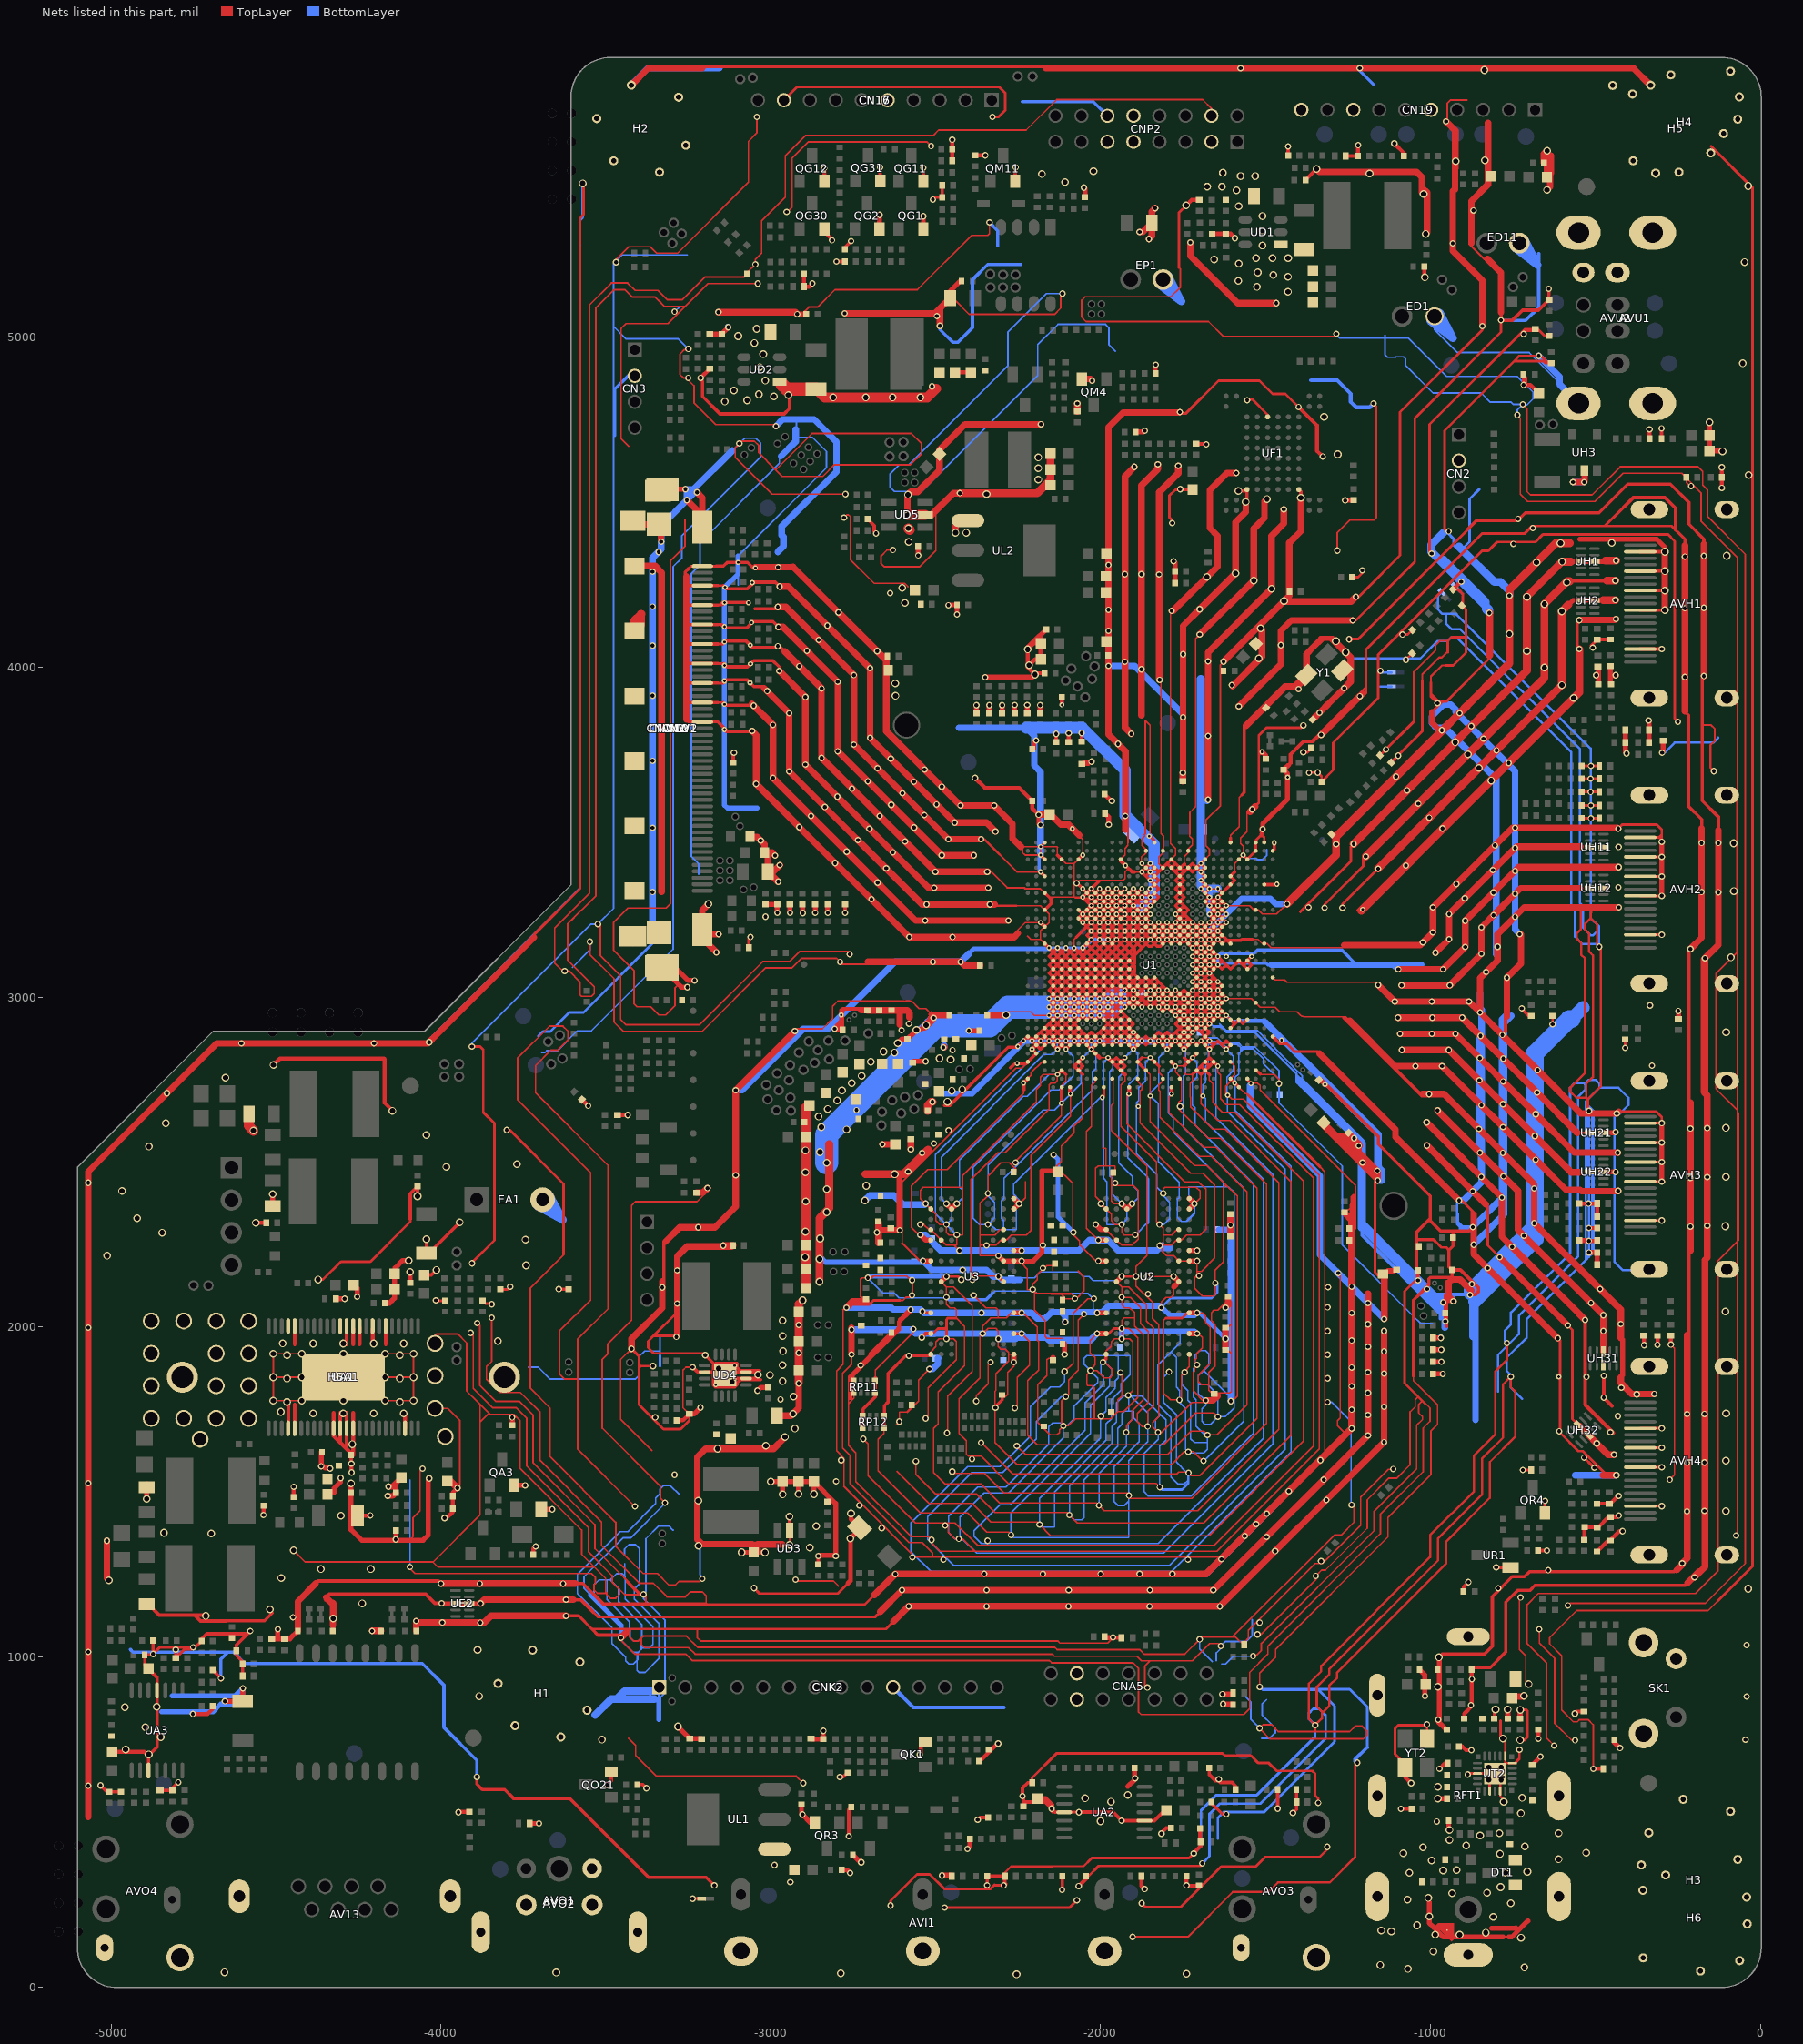
[diagram p0: the nets of this part, all layers, seen from the top]
# Altium PCB MISC86290.PcbDoc (part 17 of 31)
Units mil, origin at the board's own origin, x right, y up, seen from the top; angles counter-clockwise.
Board outline 5104.71 x 5851.49 mil, 2 copper layers (TopLayer, BottomLayer), stack 61.855 mil thick; 1026 components, 667 nets, 4280 pads, 2294 vias.

## Via types
v1: diameter 19.68, hole 11.81, TopLayer to BottomLayer, tented both sides, 1189 vias
v2: diameter 19.68/19.68 (per signal layer), hole 11.81, TopLayer to BottomLayer, tented both sides, 366 vias
v3: diameter 15.75, hole 7.87, TopLayer to BottomLayer, tented both sides, 348 vias
v4: diameter 23.62, hole 15.75, TopLayer to BottomLayer, tented both sides, 309 vias
v5: diameter 15.75/15.75 (per signal layer), hole 7.87, TopLayer to BottomLayer, tented both sides, 59 vias
v6: diameter 24/24 (per signal layer), hole 16, TopLayer to BottomLayer, tented both sides, 23 vias

## Nets (pads, with @x,y where several pads share a name; then routed paths per layer and width w, separated by ;. In a path a pad name is that pad's centre, name@x,y a point inside that pad or via, vN(x,y) a via of type N, cw(c..) or ccw(c..) an arc to the next point about the centre after c; other vN are vias at no path point) (continued)
GND: (continued)
  TopLayer w10: v1(-5032,610) -5012.67,590.67 DO32.A@-5006.75,590.67 ; DO32.A@-5008.83,590.67 DO32.A@-5006.75,590.67 ; RO40.1@-4969.75,590.67 DO32.A@-5006.75,590.67 ; CA14.2@-4892,1159.97 -4887.97,1159.97 -4854.5,1126.5 -4747,1126.5 ; UA3.10@-4886.51,638.49 UA3.10@-4886.51,655.21 -4886.51,699.26 -4887.25,700 -4860.92,726.33 UA3.4@-4860.92,898.32 -4860.92,937.73 CO41.2@-4887.19,964 -4897.27,974.08 -4897.27,1006 v1@-4875,1006 ; RO43.1@-4872.52,1053 RO43.1@-4872.52,1049 v1(-4872.52,1008.48) -4852,1029 v1(-4751.25,1029) ; DO31.A@-4851.5,594.73 RO39.1@-4813.5,594.73 -4813.5,602.63 -4796.63,619.5 v1(-4796.5,619.5) ; v1(-4804,1022) -4803.84,1021.84 CA53.1@-4803.84,996.73 -4776.57,1024 -4756.25,1024 v1(-4751.25,1029) ; v4(-4713,1124) -4715.5,1126.5 -4747,1126.5 ; CO32.1@-4691.78,959.49 -4668,935.71 -4668,930 -4667,931 v1(-4667,935) ; DE1.A@-4601,941.4 CE8.1@-4601,978.37 -4601,985.06 -4620.23,1004.29 CE7.1@-4620.23,1018.5 -4620.23,1035.77 -4586,1070 ; v1(-4578,1078) -4586,1070 ; -4511.68,1132.68 -4534.78,1109.59 -4647.98,1109.59 -4649.08,1108.5 -4729,1108.5 -4747,1126.5 ; -4379.78,1222.16 -4371.94,1230 -4007.84,1230 v2(-4000,1222.16) ; -4093,2326.45 -4093,2404.27 CA35.2@-4071,2426.27 v4(-4071,2396.54) ; CA10.1@-4051,2157.81 -4029.19,2157.81 v4(-4014,2173) ; v4(-4043.95,2265.95) CA30.1@-4043.95,2223.94 -4036.06,2223.94 v4(-3943,2317) ; v1(-3891,636) -3891,614 -3875,598 -3807,598 -3780,571 -3609.66,571 -3370.66,332 -3196.16,332 v2(-3171.25,307.09) ; v1(-3642.77,2114.77) CO24.1@-3613,2114.77 ; v2(-3621.16,1124.16) -3582.16,1124.16 -3564.25,1106.25 ; -3598,1173.16 -3576,1173.16 -3537.67,1134.83 ; -3593.16,1222.16 -3569.85,1222.16 -3507.19,1159.5 -3380.94,1159.5 -3196,1159.5 ; -3542.5,1084.5 -3524,1066 -3462.25,1066 v1(-3454.25,1058) ; v1(-3495.94,611.55) -3483.5,623.99 QO21.E@-3483.5,649.5 ; CO25.1@-3405.05,614.28 CO25.1@-3405.05,612.5 -3387.5,612.5 v1(-3377,602) v1@-3376.5,602.5 ; -3329,2138.75 -3324,2143.75 -3324,2253.75 -3319.25,2258.5 ; -3259.25,4279 -3259.25,4289.33 -3249,4299.57 ; v1(-3237.25,1878) -3222.78,1863.53 UD4.6@-3217.56,1863.53 ; v1@-3215.25,4875 -3207.5,4867.25 -3207.5,4821.44 -3154.06,4768 -2959.5,4768 -2943.5,4784 v4@-2943.5,4824.11 ; -3208,5815.96 -3203,5820.96 v1@-1575,5820.96 ; UD4.6@-3201,1863.53 -3173.28,1863.53 ; -3165,4306.65 -3143.59,4306.65 -3132.25,4318 -3113,4318 ; -3159.77,3834.21 -3130.56,3805 ; -3154.7,4188.54 -3146.25,4197 -3083.5,4197 ; -3149.74,4129.49 -3139.97,4119.72 -3072.53,4119.72 ; UD4.EPAD@-3147.85,1863.53 -3173.28,1863.53 ; -3146.81,4070.43 -3137.25,4080 -3075.25,4080 -3054.75,4059.5 ; v3@-3143.85,4247.6 -3134.08,4237.83 -3071.1,4237.83 -3050.93,4258 -3042.5,4258 ; v3@-3143.52,3893.27 -3135.25,3885 v1@-3061.25,3885 ; v3@-3143.22,3952.32 -3132.94,3962.61 -3072.64,3962.61 ; v3@-3142.63,4011.38 -3132.86,4001.61 -3070.64,4001.61 ; v3@-3141,3815.44 -3130.56,3805 ; v3(-3140.74,3811.12) -3134.62,3805 -3110,3805 ; UD4.EPAD@-3128.17,1843.85 UD4.14@-3075.02,1843.85 -3050.15,1843.85 v4(-3039,1855) -3047.53,1863.53 UD4.15@-3075.02,1863.53 UD4.15@-3089.47,1863.53 ; UD4.EPAD@-3128.17,1863.53 UD4.15@-3089.47,1863.53 ; RW415.1@-3114,3711.73 -3114,3739 v1(-3112,3741) ; v3(-3099.25,4318) -3113,4318 ; v3@-3068.25,4197 -3083.5,4197 ; v3(-3068,4195.5) -3069.5,4197 -3083.5,4197 ; RW73.2@-3066.27,3150 -3066.27,3177.23 v1(-3061.5,3182) ; v3(-3063.01,3952.99) -3072.64,3962.61 ; v3(-3062.2,4066.95) -3054.75,4059.5 ; v3(-3061.62,4010.62) -3070.64,4001.61 ; v3(-3058.19,4135.63) -3058.19,4134.06 -3072.53,4119.72 ; v1(-3057,3807) -3059,3805 -3110,3805 ; v3(-3056.37,4256.63) -3054.99,4258 -3042.5,4258 ; -3048.75,4177.5 v1@-2981.25,4177.5 ; v3(-3047,4301.5) -3045.5,4300 -3029,4300 ; -3033.2,1867.7 -3093.65,1867.7 ; -3031.17,1839.67 -3093.65,1839.67 -3102.73,1830.59 -3102.73,1825.5 -3109.82,1818.41 -3168,1818.41 -3173.28,1823.7 -3173.28,1863.53 ; -3020.25,3937 -3024.75,3941.5 -3051.53,3941.5 -3072.64,3962.61 ; v1(-2977.25,4122) -2993.75,4138.5 -3053.75,4138.5 -3072.53,4119.72 ; v1(-2974.31,3989.07) -2974.31,4000.94 -2993.87,4020.5 -3051.75,4020.5 -3070.64,4001.61 ; v1(-2973.25,4245) -2986.25,4258 -3042.5,4258 ; -2957.85,4047.4 -2969.95,4059.5 -3054.75,4059.5 ; -2932.52,4304 -2933.02,4303.5 -2936.52,4300 -3029,4300 ; v1(-2790.69,635.88) -2780.73,635.88 -2767.34,649.27 CK1.1@-2766,649.27 ; RG40.1@-2775.73,5267 -2775.73,5272.77 v1(-2756.5,5292) ; v1(-2764,456) -2764,536.98 CR5.1@-2755.98,545 ; RD55.1@-2706.7,4449.79 -2686.75,4429.83 -2686.75,4411.5 v1(-2681.25,4406) ; -2639.15,1963.32 -2612.22,1990.25 -2612.22,1998.03 ; -2622.22,1988.03 -2612.22,1998.03 ; -2607.06,2021.8 -2612.22,2016.63 -2612.22,1998.03 ; v2(-2542.64,1968.11) -2530.83,1979.92 U3.P1@-2515.08,1979.92 ; v1@-2502.16,5424.84 RG4.1@-2480.98,5424.84 CG1.1@-2480.98,5463.84 ; -2472.97,2672.03 -2457.97,2672.03 ; -2456.72,2672.03 -2280.72,2848.03 -2253.27,2848.03 v3(-2251.3,2850) v3(-2233.58,2867.72) U1.G30@-2220.79,2880.51 v3(-2207.99,2867.72) ; v1(-2373,506) -2366,513 RO30.1@-2341.73,513 ; v1(-2344.27,307.54) CI1.1@-2344.27,334.99 DI2.A@-2290.73,335 v1@-2290.73,310.35 ; v2@-2320.2,1757.54 -2298.21,1779.53 -2298.94,1780.25 C50.2@-2298.94,1787.48 ; -2273.18,2785.76 -2260.12,2798.82 -2225.71,2798.82 -2208.26,2816.26 ; v3(-2253.27,2798.82) v3@-2251.3,2796.85 ; CO18.2@-2234,546.73 -2234,559.73 ; U1.D30@-2220.79,2803.74 -2208.26,2816.26 ; RO57.1@-2207.96,618.5 -2220.82,618.5 -2237,602.32 v1(-2237,578) -2234,575 -2234,559.73 ; U1.G29@-2195.2,2880.51 U1.F28@-2169.61,2854.92 v3(-2156.81,2867.72) ; v3(-2182.4,3379.53) U1.AF28@-2169.61,3366.73 ; v3(-2182.4,3430.71) U1.AH28@-2169.61,3417.91 ; U1.H28@-2169.61,2906.1 v3(-2131.22,2867.72) ; U1.V28@-2169.61,3162.01 -2131.22,3123.62 ; U1.AB28@-2169.61,3264.37 -2150.91,3283.07 -2150.91,3294.88 -2150.91,3296.85 -2156.81,3302.76 U1.AD28@-2169.61,3315.55 ; v3@-2154.8,3147.65 -2145.22,3138.06 -2145.22,3135.22 ; -2138,529 -2148.66,539.66 -2168.73,559.73 -2234,559.73 ; v5(-2131.22,2765.35) U1.C26@-2118.43,2778.15 -2105.63,2765.35 ; -2130.79,3430.28 U1.AH26@-2118.43,3417.91 ; v3@-2129.21,3147.65 -2129.21,3147.2 -2118.43,3136.42 ; v1@-2116.54,294.46 RI4.1@-2116.54,335 ; v3@-2104,3148 -2093.13,3137.13 -2093.13,3136.13 ; -2073.84,3182.16 -2028.08,3227.92 v3@-2026.92,3227.92 ; v1(-2073.03,3344.98) -2071.09,3344.98 v3(-2054.45,3328.35) U1.AD23@-2041.65,3315.55 -1875.32,3149.21 ; U1.C24@-2067.24,2778.15 -2054.45,2790.94 U1.D24@-2067.24,2803.74 ; U1.H24@-2067.24,2906.1 v3(-2105.63,2867.72) ; U1.J24@-2067.24,2931.69 -2156.81,3021.26 U1.AE15@-1836.93,3341.14 ; U1.AB24@-2067.24,3264.37 U1.T18@-1913.7,3110.83 -1896.97,3094.09 -1896.97,3076.38 U1.P18@-1913.7,3059.65 U1.J23@-2041.65,2931.69 -2156.81,3046.85 U1.P27@-2144.02,3059.65 v3@-2054.63,3149.03 ; U1.AH24@-2067.24,3417.91 v3(-2054.45,3430.71) ; -2054.45,2765.35 -2080.04,2790.94 U1.D24@-2067.24,2803.74 ; v5(-2054.45,2816.54) U1.D24@-2067.24,2803.74 ; v3(-2054.45,3225.98) U1.AD20@-1964.88,3315.55 ; v3@-2054,3149 -2054,3148.76 -2041.62,3136.38 ; U1.AB23@-2041.65,3264.37 -1900.91,3123.62 ; -2006.88,3350.33 v3(-2028.86,3328.35) ; U1.H21@-1990.47,2906.1 v3(-1952.09,2867.72) ; U1.J21@-1990.47,2931.69 U1.P16@-1862.52,3059.65 v3(-1824.13,3021.26) ; v5(-1977.68,2816.54) -1952.09,2790.94 ; U1.D19@-1940.28,2802.76 -1952.09,2790.94 ; U1.C19@-1939.29,2778.15 -1926.5,2790.94 U1.D19@-1939.29,2803.74 ; U1.AH19@-1939.29,3417.91 -1939.29,3412.11 v3@-1926.18,3399 ; -1926.5,2765.35 -1952.09,2790.94 ; v5(-1926.5,2816.54) U1.D19@-1939.29,2803.74 ; v3(-1926.5,2970.08) U1.T24@-2067.24,3110.83 v3(-2105.63,3149.21) -2118.43,3136.42 ; v3@-1926.18,3328.03 v3(-1926.5,3328.35) U1.AD19@-1939.29,3315.55 ; v3(-1925,3399) -1924.47,3399 -1905,3379.53 -1896.81,3379.53 ; U1.P17@-1888.11,3059.65 U1.J22@-2016.06,2931.69 -2156.81,3072.44 U1.T26@-2118.43,3110.83 ; -1875.32,2816.54 U1.D17@-1888.11,2803.74 U1.C16@-1862.52,2778.15 ; v3(-1875.32,3328.35) U1.AD17@-1888.11,3315.55 ; v5(-1849.72,2816.54) U1.D15@-1836.93,2803.74 -1823.15,2789.96 ; v3(-1849.72,3225.98) -2156.81,2918.9 ; v3(-1849.72,3277.17) U1.AD17@-1888.11,3315.55 ; v3(-1849.72,3302.76) U1.AC15@-1836.93,3289.96 ; U1.G15@-1836.93,2880.51 v3(-1824.13,2867.72) ; v3(-1824.13,2970.08) U1.M13@-1785.75,3008.46 ; U1.K13@-1785.75,2957.28 v3(-1645,3098.03) ; U1.AG13@-1785.75,3392.32 -1772.95,3405.12 ; v3(-1772.95,2944.49) v3(-1670.59,3046.85) -1657.8,3059.65 ; v3(-1772.95,3225.98) v3(-1645,3098.03) ; -1747.36,2790.94 U1.D11@-1734.57,2803.74 ; -1747.36,2816.54 U1.D11@-1734.57,2803.74 ; -1746.38,3404.13 -1758.19,3392.32 U1.AG12@-1760.16,3392.32 -1772.95,3379.53 ; U1.V11@-1734.57,3162.01 v3(-1721.77,3174.8) U1.W10@-1708.98,3187.6 ; -1721.77,2765.35 U1.C10@-1708.98,2778.15 ; v3(-1721.77,2893.31) -2041.65,3213.19 ; v3(-1721.77,3149.21) U1.W9@-1683.39,3187.6 v3(-1670.59,3200.39) ; v3(-1721.77,3225.98) U1.V13@-1785.75,3162.01 U1.AD19@-1939.29,3315.55 ; CF1.1@-1710.27,4677 v1@-1681,4677 ; U1.E10@-1708.98,2829.33 v5(-1721.77,2816.54) U1.D11@-1734.57,2803.74 ; v3(-1696.18,3379.53) U1.AG9@-1683.39,3392.32 v3(-1696.18,3405.12) ; U1.T9@-1683.39,3110.83 -1682.94,3110.83 v3@-1670.59,3123.18 ; U1.AE9@-1683.39,3341.14 v3(-1696.18,3328.35) U1.AD9@-1683.39,3315.55 ; U1.AH9@-1683.39,3417.91 -1721.77,3379.53 U1.AG11@-1734.57,3392.32 ; CO11.1@-1671.5,663.02 -1671.5,644 -1651,623.5 v1@-1642,623.5 ; -1669.61,2764.37 U1.C9@-1683.39,2778.15 ; RO58.1@-1664.77,555.5 -1664,555.5 -1631.5,523 v1(-1619.5,523) ; U1.R8@-1657.8,3085.24 v3(-1798.54,3225.98) -1875.32,3149.21 ; U1.V8@-1657.8,3162.01 -1734.57,3238.78 ; -1656,628.5 v1(-1642,628.5) v1@-1642,623.5 ; v5(-1645,2790.94) U1.D8@-1657.8,2803.74 ; v3(-1645,3328.35) U1.AD7@-1632.2,3315.55 ; U1.K7@-1632.2,2957.28 v3(-1645,2944.49) U1.J8@-1657.8,2931.69 ; v5(-1619.41,2842.13) -1632.52,2855.24 ; v3(-1619.41,2944.49) v3(-1721.77,3046.85) v3(-1645,3123.62) ; U1.AE6@-1608.58,3339.17 -1593.82,3353.94 U1.AF6@-1606.61,3366.73 ; U1.B6@-1606.61,2752.56 v5(-1593.82,2739.76) U1.A5@-1581.02,2726.97 ; U1.F6@-1606.61,2854.92 -1617.72,2866.03 -1619.41,2867.72 -1631.89,2855.24 -1632.52,2855.24 ; U1.H6@-1606.61,2906.1 -1593.82,2918.9 ; U1.J6@-1606.61,2931.69 -1593.82,2918.9 ; U1.V6@-1606.61,3162.01 -1619.41,3174.8 ; U1.AE6@-1606.61,3341.14 U1.AD7@-1632.2,3315.55 ; U1.AK6@-1606.61,3469.09 -1606.61,3482 ; U1.AF6@-1604.65,3368.7 -1594.31,3379.04 ; CO16.1@-1591.54,597.85 -1591.54,609.14 -1601.56,619.16 -1637.66,619.16 v1@-1642,623.5 ; v4(-1582.27,4534.76) -1560.63,4534.76 UF1.K3@-1556.74,4538.65 v4@-1556.74,4502.62 ; -1572.32,3174.8 -1574.73,3172.4 ; -1572.03,3613.73 -1564.47,3621.28 -1564.47,3817.66 -1559.47,3822.66 ; U1.J4@-1556.42,2931.69 -1568.72,2919.39 U1.J5@-1581.02,2931.69 -1593.82,2918.9 ; v3(-1542.64,3123.62) U1.T4@-1555.43,3110.83 ; -1539.7,3174.8 -1556.98,3174.8 -1557.05,3174.87 -1572.25,3174.87 -1574.73,3172.4 ; U1.C3@-1529.84,2778.15 -1527.64,2778.15 -1517.05,2767.56 ; U1.AE2@-1504.25,3341.14 -1465.87,3341.14 v3(-1465.87,3342.13) ; U1.G1@-1478.66,2880.51 -1457.5,2859.35 -1441,2859.35 ; U1.AJ1@-1478.66,3443.5 -1474,3448.17 v3(-1474,3468.11) ; v1(-1463.54,539.91) CO12.1@-1463.54,597.85 ; v1(-1417.5,526.5) -1406.73,537.27 DO11.A@-1406.73,559.5 RO24.1@-1406.73,597.46 ; UF1.K8@-1399.26,4538.65 -1393.25,4532.64 v4(-1393.25,4514.11) ; -1357.22,3776.78 v1@-1339,3795 ; v3@-1322.64,2741.47 -1158.5,2577.33 -1158.5,2554.71 -1001,2397.21 -1001,2322.09 -970.07,2291.16 -883.84,2291.16 v1(-872,2303) ; v3@-1320.97,2736.05 -1320.46,2735.54 v3(-1320.46,2735.22) ; -1262.64,2937.08 -1026.72,2701.16 ; C201.1@-1143.1,2160.9 -1130.73,2173.27 C205.1@-1103,2173.27 -1112.27,2164 C201.1@-1132,2164 ; v1(-1090,539) CT26.1@-1057.73,539 ; -1085,2759.44 -1026.72,2701.16 ; -1052,1851 -1052,2081.05 -1033.05,2100 ; DO2.A@-1043,2171.54 -1043,2269.5 ; DO2.A@-1038.96,2167.5 -1038.96,2142.46 v1(-1038,2141.5) ; -1018.5,2701.16 -1026.72,2701.16 ; v1(-1011,2115) -1018.05,2115 -1033.05,2100 ; -1001,2329 -1043,2287 -1043,2269.5 ; -986.67,2261.02 -990.81,2265.16 -1038.66,2265.16 -1043,2269.5 ; v4(-975,998.5) -965,1008.5 -836.27,1008.5 -812.81,1031.96 -812.81,1182.67 -752.48,1243 ; v1(-955.2,2017.2) C30.1@-955.2,2042.53 ; v1@-955.2,2017.7 C30.1@-955.2,2042.53 ; v1@-955.2,2078.13 v1(-930.63,2078.13) ; -955.2,2095.63 C30.1@-955.2,2042.53 ; -951,2002 -951,2138.27 ; -944.34,2230.16 -944.34,2220 ; -941.59,2150.17 -1001.04,2150.17 -1005.16,2146.05 -1005.16,2127.9 -1033.05,2100 ; -935.04,2144.06 RO2.1@-935.04,2173 ; -932.04,2290.13 R151.2@-932.04,2271.3 -932.04,2245.68 -944.34,2233.37 -944.34,2220 ; CR2.1@-899.73,1198 -899.73,1212.27 v1(-885.5,1226.5) ; -886.6,4419.31 -860.91,4445 -859.49,4445 -736,4445 v1@-731,4450 ; v1(-880.5,2097.5) -865.09,2097.5 -854.39,2108.19 -854.39,2117.95 -909.44,2173 RO2.1@-935.04,2173 ; CT21.2@-871.14,967.5 -819.28,967.5 -771.81,1014.97 -771.81,1165.69 -735.5,1202 -698.35,1202 -683.6,1216.75 -228.25,1216.75 -176.16,1268.84 ; -843.25,5075.42 -843.25,5099.2 ; v1(-800.9,1271.1) UR1.1@-757.26,1271.1 ; v1(-786.25,5052) -751.84,5052 -721.34,5082.5 -672.58,5082.5 -656.22,5098.86 -655.85,5098.86 -641.5,5113.21 v1(-641.5,5147.5) ; v1@-786.25,5060 -786.25,5075.59 ; v1(-782.46,2885.54) -772.84,2895.16 -772.84,2959.42 -770.63,2961.63 ; v1(-734.5,4450) v1@-731,4450 ; -730,1243 -752.48,1243 ; v1(-723.5,2966) -723.5,2964.5 -702.27,2943.27 D40.A@-695,2943.27 ; RR19.2@-674.04,1322.5 v1(-647.5,1322.5) ; -655,4468.2 -672.72,4468.2 ; QR4.E@-653.1,1436 v1(-653.1,1472.4) ; v1(-643.12,1262.59) v1@-638.28,1257.75 ; v4@-578.25,4261 -468.2,4261 ; v1@-556,4052 -556,4120 ; v1(-549,4143) -556,4136 -556,4120 ; v1@-542.25,4143.87 -549.13,4143.87 -556,4137 -556,4120 ; v1(-508.5,4059.5) -512.5,4063.5 -512.5,4065.77 CH6.2@-495,4083.27 ; v1(-506.83,660.5) DR2.A@-476.23,660.5 ; CH6.2@-494,4084.27 DH5.A@-456,4084.27 ; -447,4453 -385.5,4514.5 -289.5,4514.5 -257.5,4482.5 -257.5,4416.59 ; AVH1.11@-365.72,4173.23 v4(-289.88,4173.23) ; AVH1.8@-365.72,4232.29 v4(-289.88,4232.29) ; AVH1.5@-365.72,4291.34 v4(-289.88,4291.34) ; AVH1.2@-365.72,4350.4 v4(-289.88,4350.4) ; AVH1.17@-364.47,4055.12 v1@-299.12,4055.12 ; -246.95,4406.05 -229,4388.09 -229,4370 ; v1(-237,1284) -263.25,1257.75 v1@-638.28,1257.75 ; -229,3866.1 -217.5,3854.6 -217.5,3578.43 -178,3538.93 -178,3503.33 ; -217.16,1976.09 v1@-217.16,3148.02 ; v1@-176.5,3968.5 -176.5,3825 -176.5,3595.41 -127.5,3546.41 -127.5,3506.5 ; -171.5,4373 -171.5,4388.57 -216.5,4433.57 -216.5,4499.48 -272.52,4555.5 -402.48,4555.5 -489.78,4468.2 -672.72,4468.2 ; v1(-4751.25,1029) -4744.25,1029 CO31.1@-4725.25,1048 -4725.25,1054.92 -4710.16,1070 -4586,1070 ; -3173.28,1863.53 -3173.28,1882.5 -3170.05,1885.73 -3166.82,1888.96 -3103,1888.96 -3102.73,1888.7 -3102.73,1876.79 -3093.65,1867.7 ; -3130.56,3805 -3110,3805 ; -3113,4318 -3070.45,4318 -3052.45,4300 -3029,4300 ; -3093.65,1867.7 UD4.15@-3089.47,1863.53 ; -2208.26,2816.26 U1.E29@-2195.2,2829.33 v3(-2207.99,2842.13) v3(-1824.13,3225.98) U1.Y14@-1811.34,3213.19 U1.V12@-1760.16,3162.01 v3(-1696.18,3225.98) U1.Y9@-1683.39,3213.19 ; v3(-2207.99,2867.72) -2182.4,2842.13 v3(-2156.81,2867.72) ; v3(-2207.99,2867.72) -2182.4,2893.31 ; -2182.4,2893.31 -2156.81,2918.9 ; -2182.4,2893.31 v3(-2156.81,2867.72) ; v3(-2156.81,2867.72) v5(-2131.22,2842.13) v3(-2105.63,2867.72) ; v3(-2156.81,2867.72) U1.F27@-2144.02,2854.92 v3(-2131.22,2867.72) ; v3(-2156.81,2867.72) -1900.91,3123.62 ; -2156.81,2918.9 v3(-2105.63,2867.72) ; -2145.22,3135.22 -2156.81,3123.62 U1.T27@-2144.02,3110.83 U1.G18@-1913.7,2880.51 ; -2145.22,3135.22 v3(-2131.22,3149.21) U1.T25@-2092.83,3110.83 -1926.5,2944.49 ; U1.K27@-2144.02,2957.28 v3(-2054.45,2867.72) ; U1.K27@-2144.02,2957.28 v3(-2156.81,2944.49) v3(-2080.04,2867.72) ; U1.K27@-2144.02,2957.28 v3(-2156.81,2970.08) U1.AC15@-1836.93,3289.96 ; U1.K27@-2144.02,2957.28 U1.AA16@-1862.52,3238.78 v3(-1849.72,3251.57) U1.AB16@-1862.52,3264.37 U1.AD18@-1913.7,3315.55 ; v3(-2131.22,2867.72) U1.F26@-2118.43,2854.92 v3(-2105.63,2867.72) ; v3(-2131.22,2867.72) v5(-2105.63,2842.13) -2087.22,2860.53 ; v3(-2131.22,2867.72) U1.R18@-1913.7,3085.24 -1896.97,3101.97 -1896.97,3145.28 -2041.65,3289.96 ; -2131.22,3123.62 -2156.81,3098.03 U1.R27@-2144.02,3085.24 v3(-1926.5,2867.72) ; -2131.22,3123.62 U1.T26@-2118.43,3110.83 ; -2131.22,3123.62 -2118.43,3136.42 ; U1.T26@-2118.43,3110.83 U1.H18@-1913.7,2906.1 ; U1.T26@-2118.43,3110.83 -2093.13,3136.13 ; v3(-2105.63,2867.72) U1.F25@-2092.83,2854.92 -2087.22,2860.53 ; -2093.13,3136.13 -2080.04,3149.21 v3(-1900.91,2970.08) -1824.13,3046.85 ; -2087.22,2860.53 v3(-2080.04,2867.72) ; v3(-2080.04,2867.72) U1.F24@-2067.24,2854.92 v3(-2054.45,2867.72) ; v3(-2080.04,2867.72) -2054.45,2893.31 ; v3@-2054.63,3149.03 -2054.27,3149.03 -2041.62,3136.38 ; v3@-2054.63,3149.03 U1.V23@-2041.65,3162.01 ; v3(-2054.45,2867.72) U1.F23@-2041.65,2854.92 ; v3(-2054.45,2867.72) -2028.86,2893.31 v3(-2003.27,2867.72) ; -2054.45,2893.31 v3(-2156.81,2995.67) U1.AD15@-1836.93,3315.55 ; -2054.45,2893.31 v3(-2028.86,2867.72) ; U1.F23@-2041.65,2854.92 U1.F23@-2040.72,2853.99 ; U1.F23@-2041.65,2854.92 U1.F23@-2041.13,2855.44 ; U1.V23@-2041.65,3162.01 v3(-1849.72,2970.08) U1.M14@-1811.34,3008.46 ; U1.V23@-2041.65,3162.01 U1.AD17@-1888.11,3315.55 ; -2041.65,3213.19 U1.AA24@-2067.24,3238.78 U1.AD21@-1990.47,3315.55 ; -2041.65,3213.19 v3@-2026.92,3227.92 ; -2041.65,3289.96 v3(-2054.45,3302.76) v3(-2028.86,3328.35) ; -2041.65,3289.96 U1.AD22@-2016.06,3315.55 v3(-2003.27,3328.35) U1.AD21@-1990.47,3315.55 ; -2041.62,3136.38 v3(-1875.32,2970.08) v3(-1824.13,3021.26) ; U1.F23@-2041.13,2855.44 -2040.72,2855.03 U1.F23@-2040.72,2853.99 ; U1.F23@-2041.13,2855.44 v3(-2028.86,2867.72) ; U1.F23@-2040.72,2853.99 v5(-2028.86,2842.13) -2009.34,2861.65 ; v3(-2028.86,2867.72) U1.F22@-2016.06,2854.92 -2009.34,2861.65 ; v3(-2028.86,2867.72) -2003.27,2893.31 ; v3(-2028.86,3328.35) -1854.65,3154.13 -1844.8,3154.13 v3(-1824.13,3174.8) U1.AA12@-1760.16,3238.78 ; v3@-2026.92,3227.92 U1.AD19@-1939.29,3315.55 ; -2009.34,2861.65 v3(-2003.27,2867.72) ; v3(-2003.27,2867.72) U1.F21@-1990.47,2854.92 -1977.68,2867.72 ; v3(-2003.27,2867.72) U1.J19@-1939.29,2931.69 -1926.5,2944.49 ; -2003.27,2893.31 -1977.68,2867.72 ; -2003.27,2893.31 U1.P15@-1836.93,3059.65 -1824.13,3046.85 ; U1.AD21@-1990.47,3315.55 v3(-1849.72,3174.8) -1829.06,3154.13 -1819.21,3154.13 U1.V14@-1811.34,3162.01 ; U1.AD21@-1990.47,3315.55 v3(-1977.68,3328.35) U1.AD20@-1964.88,3315.55 ; -1977.68,2867.72 U1.F20@-1964.88,2854.92 v3(-1952.09,2867.72) ; -1977.68,2867.72 U1.J18@-1913.7,2931.69 ; U1.AD20@-1964.88,3315.55 U1.V14@-1811.34,3162.01 ; U1.AD20@-1964.88,3315.55 v3(-1952.09,3328.35) U1.AD19@-1939.29,3315.55 ; -1952.09,2790.94 U1.D20@-1964.88,2803.74 -1952.09,2816.54 U1.D19@-1939.29,2803.74 ; v3(-1952.09,2867.72) U1.F19@-1939.29,2854.92 v3(-1926.5,2867.72) ; v3(-1952.09,2867.72) U1.H18@-1913.7,2906.1 ; v3(-1926.5,2867.72) U1.F18@-1913.7,2854.92 ; v3(-1926.5,2867.72) U1.G18@-1913.7,2880.51 ; -1926.5,2944.49 U1.J18@-1913.7,2931.69 ; U1.F18@-1913.7,2854.92 v5(-1900.91,2842.13) U1.F17@-1888.11,2854.92 ; U1.F18@-1913.7,2854.92 v3(-1900.91,2867.72) ; U1.G18@-1913.7,2880.51 v3(-1900.91,2867.72) ; U1.G18@-1913.7,2880.51 v3(-1900.91,2893.31) ; U1.H18@-1913.7,2906.1 v3(-1900.91,2893.31) ; U1.H18@-1913.7,2906.1 -1900.91,2918.9 U1.J18@-1913.7,2931.69 ; U1.AD18@-1913.7,3315.55 -2041.65,3187.6 U1.K14@-1811.34,2957.28 -1747.36,3021.26 U1.M11@-1734.57,3008.46 v3(-1721.77,2995.67) -1708.98,2982.87 ; U1.AD18@-1913.7,3315.55 v3(-1900.91,3328.35) U1.AD17@-1888.11,3315.55 ; v3(-1900.91,2867.72) U1.F17@-1888.11,2854.92 ; v3(-1900.91,2867.72) U1.G17@-1888.11,2880.51 ; v3(-1900.91,2893.31) U1.G17@-1888.11,2880.51 ; -1900.91,3123.62 -1875.32,3149.21 ; U1.F17@-1888.11,2854.92 v3(-1875.32,2867.72) ; U1.G17@-1888.11,2880.51 v3(-1875.32,2867.72) ; v3(-1875.32,2867.72) -1862.52,2854.92 v3(-1849.72,2867.72) ; v3(-1875.32,2867.72) -1862.52,2880.51 v3(-1849.72,2867.72) ; -1862.52,3366.73 U1.AG15@-1836.93,3392.32 ; -1862.52,3366.73 v3(-1875.32,3379.53) U1.AG16@-1862.52,3392.32 ; -1862.52,3366.73 v3(-1849.72,3353.94) ; U1.AG16@-1862.52,3392.32 U1.AF15@-1836.93,3366.73 ; U1.AG16@-1862.52,3392.32 v3(-1849.72,3405.12) U1.AG15@-1836.93,3392.32 ; v3(-1849.72,2867.72) U1.F15@-1836.93,2854.92 v3(-1824.13,2867.72) ; v3(-1849.72,2867.72) -1824.13,2893.31 v3(-1798.54,2867.72) ; v3(-1849.72,3353.94) U1.AE15@-1836.93,3341.14 ; v3(-1849.72,3353.94) U1.AF15@-1836.93,3366.73 ; U1.AC15@-1836.93,3289.96 -1824.13,3302.76 U1.AD15@-1836.93,3315.55 ; U1.AD15@-1836.93,3315.55 -1824.13,3328.35 U1.AE15@-1836.93,3341.14 ; U1.AE15@-1836.93,3341.14 -1824.13,3353.94 U1.AF15@-1836.93,3366.73 ; U1.AF15@-1836.93,3366.73 -1824.13,3379.53 ; U1.AG15@-1836.93,3392.32 -1824.13,3379.53 ; v3(-1824.13,2867.72) U1.F14@-1811.34,2854.92 ; v3(-1824.13,2867.72) -1798.54,2893.31 v3(-1772.95,2867.72) ; v3(-1824.13,3021.26) U1.M14@-1811.34,3008.46 ; v3(-1824.13,3021.26) -1811.34,3034.06 ; -1824.13,3046.85 -1811.34,3034.06 ; -1824.13,3379.53 U1.AG14@-1811.34,3392.32 -1798.54,3405.12 ; U1.F14@-1811.34,2854.92 v5(-1798.54,2842.13) -1780.18,2860.49 ; U1.F14@-1811.34,2854.92 v3(-1798.54,2867.72) ; U1.M14@-1811.34,3008.46 v3(-1721.77,2918.9) ; U1.M14@-1811.34,3008.46 v3(-1798.54,3021.26) ; -1811.34,3034.06 v3(-1798.54,3021.26) ; U1.V14@-1811.34,3162.01 -1734.57,3238.78 ; v3(-1798.54,2867.72) U1.F13@-1785.75,2854.92 -1780.18,2860.49 ; v3(-1798.54,2867.72) -1772.95,2893.31 ; v3(-1798.54,3021.26) U1.M13@-1785.75,3008.46 ; -1798.54,3405.12 -1772.95,3379.53 ; -1798.54,3405.12 U1.AH13@-1785.75,3417.91 -1772.95,3405.12 ; U1.M13@-1785.75,3008.46 v3(-1772.95,2995.67) -1760.16,2982.87 v3(-1747.36,2970.08) -1734.57,2957.28 ; U1.M13@-1785.75,3008.46 v3(-1772.95,3021.26) U1.M12@-1760.16,3008.46 v3(-1747.36,2995.67) U1.L11@-1734.57,2982.87 v3(-1721.77,2970.08) ; -1780.18,2860.49 v3(-1772.95,2867.72) ; v3(-1772.95,2867.72) U1.G12@-1760.16,2880.51 v3(-1747.36,2893.31) U1.H11@-1734.57,2906.1 v3(-1721.77,2918.9) ; v3(-1772.95,2867.72) U1.F12@-1760.16,2854.92 ; -1772.95,2893.31 -1760.16,2906.1 v3(-1747.36,2918.9) U1.J11@-1734.57,2931.69 ; -1772.95,2893.31 v3(-1747.36,2867.72) ; -1772.95,3379.53 -1747.36,3353.94 -1772.95,3328.35 -1747.36,3302.76 -1772.95,3277.17 U1.AB12@-1760.16,3264.37 -1747.36,3251.57 ; -1772.95,3405.12 -1747.36,3379.53 ; U1.F12@-1760.16,2854.92 v5(-1747.36,2842.13) -1728.09,2861.4 ; U1.F12@-1760.16,2854.92 v3(-1747.36,2867.72) ; U1.AA12@-1760.16,3238.78 -1747.36,3251.57 ; U1.AA12@-1760.16,3238.78 v3(-1772.95,3251.57) -1747.36,3277.17 ; U1.AA12@-1760.16,3238.78 v3(-1747.36,3225.98) U1.Y11@-1734.57,3213.19 v3(-1721.77,3200.39) U1.W10@-1708.98,3187.6 ; v3(-1747.36,2867.72) U1.H10@-1708.98,2906.1 ; v3(-1747.36,2867.72) U1.F11@-1734.57,2854.92 -1728.09,2861.4 ; -1747.36,3251.57 -1734.57,3238.78 ; -1747.36,3251.57 -1734.57,3264.37 -1747.36,3277.17 ; -1747.36,3277.17 -1772.95,3302.76 -1747.36,3328.35 -1772.95,3353.94 -1747.36,3379.53 ; -1747.36,3379.53 U1.AG11@-1734.57,3392.32 ; U1.J11@-1734.57,2931.69 v3(-1721.77,2944.49) ; U1.J11@-1734.57,2931.69 v3(-1721.77,2918.9) ; -1734.57,2957.28 v3(-1721.77,2970.08) ; -1734.57,2957.28 v3(-1747.36,2944.49) U1.J12@-1760.16,2931.69 -1772.95,2918.9 v3(-1721.77,2867.72) ; -1734.57,2957.28 v3(-1721.77,2944.49) ; U1.AG11@-1734.57,3392.32 -1721.77,3405.12 U1.AF9@-1683.39,3366.73 v3(-1696.18,3353.94) v3(-1670.59,3328.35) U1.AD9@-1683.39,3315.55 ; -1728.09,2861.4 v3(-1721.77,2867.72) ; v3(-1721.77,2867.72) U1.F10@-1708.98,2854.92 v3(-1696.18,2867.72) ; v3(-1721.77,2918.9) U1.H10@-1708.98,2906.1 ; v3(-1721.77,2918.9) U1.J10@-1708.98,2931.69 ; v3(-1721.77,2944.49) U1.J10@-1708.98,2931.69 ; v3(-1721.77,2944.49) -1708.98,2957.28 ; v3(-1721.77,2970.08) -1708.98,2982.87 ; v3(-1721.77,2970.08) -1708.98,2957.28 ; U1.C10@-1708.98,2778.15 -1696.18,2765.35 U1.C9@-1683.39,2778.15 ; U1.C10@-1708.98,2778.15 -1696.18,2790.94 ; U1.H10@-1708.98,2906.1 -1696.18,2893.31 ; U1.H10@-1708.98,2906.1 v3(-1696.18,2918.9) ; U1.J10@-1708.98,2931.69 v3(-1696.18,2918.9) ; U1.J10@-1708.98,2931.69 v3(-1696.18,2944.49) ; -1708.98,2957.28 v3(-1696.18,2944.49) ; -1708.98,2957.28 v3(-1696.18,2970.08) ; -1708.98,2982.87 v3(-1696.18,2995.67) v3(-1670.59,3021.26) v3(-1645,3046.85) ; -1708.98,2982.87 v3(-1696.18,2970.08) ; U1.W10@-1708.98,3187.6 v3(-1696.18,3200.39) U1.Y9@-1683.39,3213.19